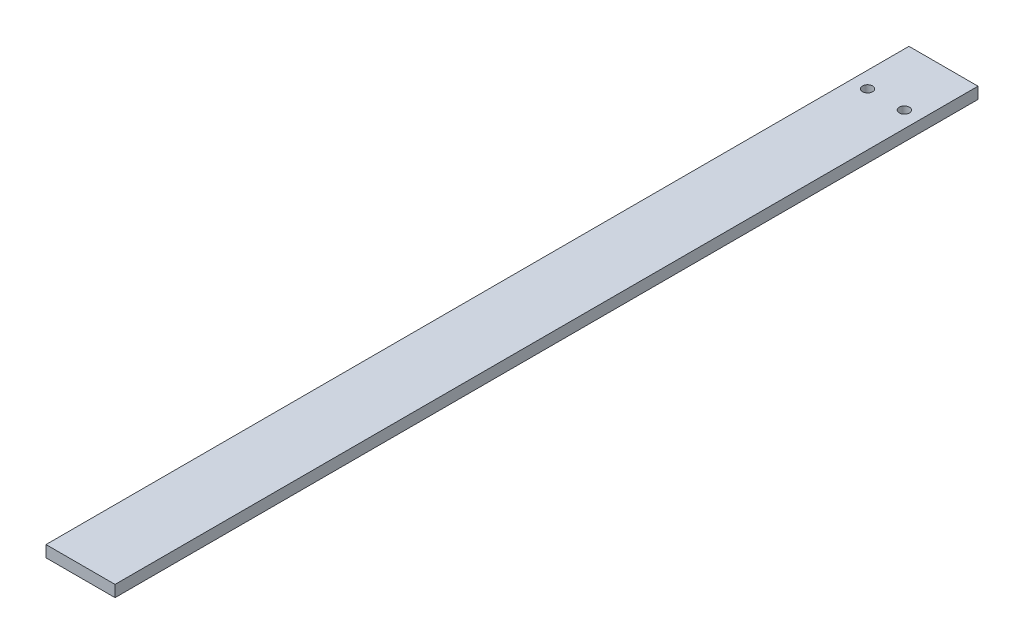
from build123d import *

# Parameters (mm, degrees)
SKETCH_1_W          = 30
SKETCH_1_H          = 5
EXTRUDE_1_DEPTH     = 15
SKETCH_2_W          = 30
SKETCH_2_H          = 10
EXTRUDE_2_DEPTH     = 172.5
SKETCH_3_R          = 2.2
CUT_EXTRUDE_1_DEPTH = 10
SKETCH_4_W          = 30
SKETCH_4_H          = 2.5
EXTRUDE_3_DEPTH     = 15
SKETCH_5_W          = 30
SKETCH_5_H          = 2.5
EXTRUDE_4_DEPTH     = 15
SKETCH_6_W          = 30
SKETCH_6_H          = 375
CUT_EXTRUDE_2_DEPTH = 5


with BuildPart() as part:
    # 草图1 → 凸台-拉伸1 (new body)
    with BuildSketch(Plane.XY):
        Rectangle(SKETCH_1_W, SKETCH_1_H)
    extrude(amount=EXTRUDE_1_DEPTH)

    # 草图2 → 凸台-拉伸2 (add)
    with BuildSketch(Plane(origin=(0, 0, 0), x_dir=(-1, 0, 0), z_dir=(0, 0, -1))):
        Rectangle(SKETCH_2_W, SKETCH_2_H)
    extrude(amount=EXTRUDE_2_DEPTH)

    # 镜向2: part across plane


with BuildPart() as part_1:
    add(part.part)
    add(part.part.mirror(Plane(origin=(0, 0, -172.5), x_dir=(1, 0, 0), z_dir=(0, 0, -1))))

    # 草图3 → 切除-拉伸1 (cut)
    with BuildSketch(Plane(origin=(0, 5, 0), x_dir=(1, 0, 0), z_dir=(0, 1, 0))):
        with Locations(Location((8, 335, 0), (0, 0, 270))):
            Circle(SKETCH_3_R)
        with Locations(Location((-8, 335, 0), (0, 0, 270))):
            Circle(SKETCH_3_R)
    extrude(amount=-CUT_EXTRUDE_1_DEPTH, mode=Mode.SUBTRACT)

    # 草图4 → 凸台-拉伸3 (add)
    with BuildSketch(Plane(origin=(0, 0, -345), x_dir=(-1, 0, 0), z_dir=(0, 0, -1))):
        with Locations((0, 3.75)):
            Rectangle(SKETCH_4_W, SKETCH_4_H)
        with Locations((0, -3.75)):
            Rectangle(SKETCH_4_W, SKETCH_4_H)
    extrude(amount=EXTRUDE_3_DEPTH)

    # 草图5 → 凸台-拉伸4 (add)
    with BuildSketch(Plane.XY):
        with Locations((0, 3.75)):
            Rectangle(SKETCH_5_W, SKETCH_5_H)
        with Locations((0, -3.75)):
            Rectangle(SKETCH_5_W, SKETCH_5_H)
    extrude(amount=EXTRUDE_4_DEPTH)

    # 草图6 → 切除-拉伸2 (cut)
    with BuildSketch(Plane(origin=(0, 5, 0), x_dir=(1, 0, 0), z_dir=(0, 1, 0))):
        with Locations((0, 172.5)):
            Rectangle(SKETCH_6_W, SKETCH_6_H)
    extrude(amount=-CUT_EXTRUDE_2_DEPTH, mode=Mode.SUBTRACT)


solid = part_1.part
